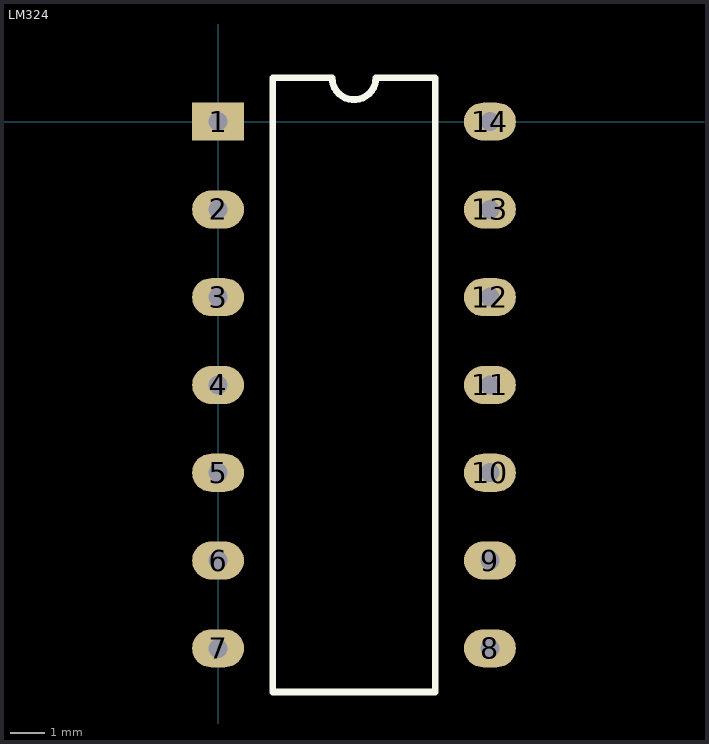
[diagram p0: the footprints below, top view; thin cyan lines are the x and y axes]
# Altium footprint library MISC89340-9.PcbLib: 4 footprints
Each footprint in its own frame and in the unit in brackets; x right, y up, seen from the top. Pads: shape width x height; smd on the part's side, far side on the other; paste and mask are expansions set on the pad; w line width, h text height; cw(c..) or ccw(c..) is an arc to the next point about the centre after c.

## LM324 [mm]
pads (14):
  rect 1.5x1.1 hole 0.55: 1(0,0)
  oval 1.5x1.1 hole 0.55: 2(0,-2.54) 3(0,-5.08) 4(0,-7.62) 5(0,-10.16) 6(0,-12.7) 7(0,-15.24) 8(7.87,-15.24) 9(7.87,-12.7) 10(7.87,-10.16) 11(7.87,-7.62) 12(7.87,-5.08) 13(7.87,-2.54) 14(7.87,0)
Top Overlay:
  lines w0.2: 1.585,-16.51 1.585,1.27 3.3,1.27 ccw(c3.935,1.27) 4.57,1.27 6.285,1.27 6.285,-16.51 1.585,-16.51

## PCBComponent_1 [mm]

## PCBComponent_1 - duplicate [mm]

## PCBComponent_1 - duplicate1 [mm]